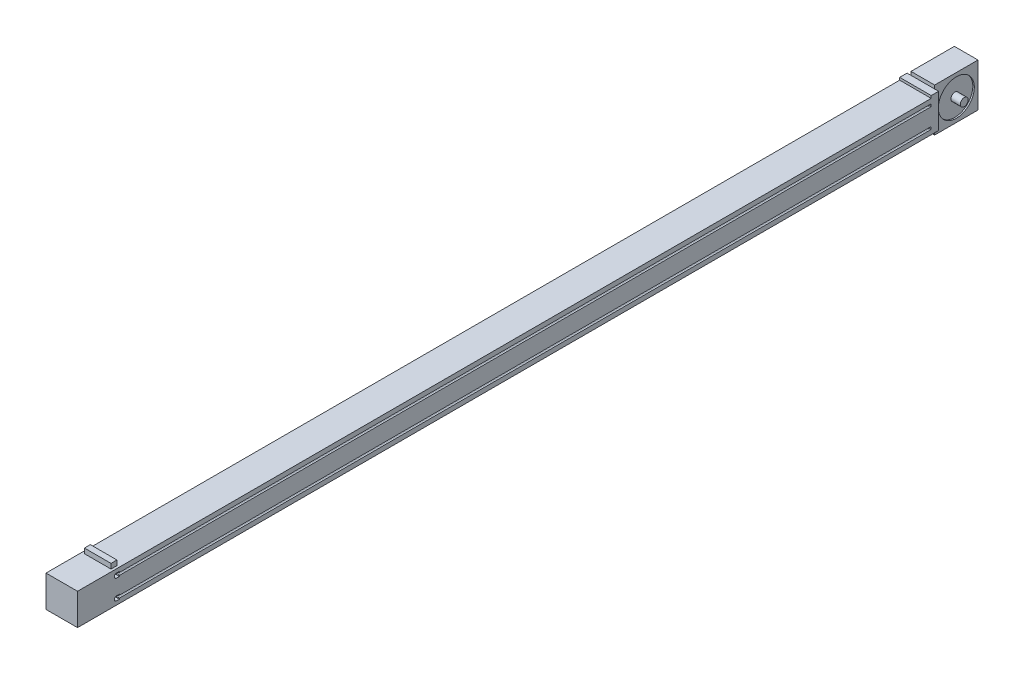
SolidWorks part; units mm, degrees
ref_plane "前视" through (0, 0, 0) normal (0, 0, 1) x (1, 0, 0)
ref_plane "上视" through (0, 0, 0) normal (0, 1, 0) x (1, 0, 0)
ref_plane "右视" through (0, 0, 0) normal (1, 0, 0) x (0, 0, -1)
sketch "草图1" plane through (0, 0, 0) normal (0, 0, 1) x (1, 0, 0)
  line L0 (41.9319, 63.6353) -> (41.9319, -24.9145) construction
  line L1 (9.9319, 6.9259) -> (9.9319, 41.9259)
  line L2 (9.9319, 56.4259) -> (73.9319, 56.4259)
  line L3 (9.9319, 46.9259) -> (12.9319, 46.9259)
  line L4 (1.2009, 24.4259) -> (59.3506, 24.4259) construction
  line L5 (12.9319, 46.9259) -> (12.9319, 48.4259)
  line L6 (12.9319, 48.4259) -> (16.9319, 48.4259)
  line L7 (16.9319, 48.4259) -> (16.9319, 40.4259)
  line L8 (16.9319, 40.4259) -> (12.9319, 40.4259)
  line L9 (12.9319, 40.4259) -> (12.9319, 41.9259)
  line L10 (12.9319, 41.9259) -> (9.9319, 41.9259)
  line L11 (9.9319, 46.9259) -> (9.9319, 56.4259)
  line L12 (9.9319, 1.9259) -> (9.9319, -7.5741)
  line L13 (12.9319, 6.9259) -> (9.9319, 6.9259)
  line L14 (12.9319, 8.4259) -> (12.9319, 6.9259)
  line L15 (16.9319, 8.4259) -> (12.9319, 8.4259)
  line L16 (16.9319, 0.4259) -> (16.9319, 8.4259)
  line L17 (12.9319, 0.4259) -> (16.9319, 0.4259)
  line L18 (12.9319, 1.9259) -> (12.9319, 0.4259)
  line L19 (9.9319, 1.9259) -> (12.9319, 1.9259)
  line L20 (9.9319, -7.5741) -> (73.9319, -7.5741)
  line L21 (73.9319, 1.9259) -> (70.9319, 1.9259)
  line L22 (70.9319, 1.9259) -> (70.9319, 0.4259)
  line L23 (70.9319, 0.4259) -> (66.9319, 0.4259)
  line L24 (66.9319, 0.4259) -> (66.9319, 8.4259)
  line L25 (66.9319, 8.4259) -> (70.9319, 8.4259)
  line L26 (70.9319, 8.4259) -> (70.9319, 6.9259)
  line L27 (70.9319, 6.9259) -> (73.9319, 6.9259)
  line L28 (73.9319, 1.9259) -> (73.9319, -7.5741)
  line L29 (73.9319, 46.9259) -> (73.9319, 56.4259)
  line L30 (70.9319, 41.9259) -> (73.9319, 41.9259)
  line L31 (70.9319, 40.4259) -> (70.9319, 41.9259)
  line L32 (66.9319, 40.4259) -> (70.9319, 40.4259)
  line L33 (66.9319, 48.4259) -> (66.9319, 40.4259)
  line L34 (70.9319, 48.4259) -> (66.9319, 48.4259)
  line L35 (70.9319, 46.9259) -> (70.9319, 48.4259)
  line L36 (73.9319, 46.9259) -> (70.9319, 46.9259)
  line L37 (73.9319, 6.9259) -> (73.9319, 41.9259)
  point P25 (9.9319, 24.4259)
  point P26 (41.9319, -7.5741)
  point P43 (41.9319, 56.4259)
  dimension "D1" = 32
  dimension "D2" = 32
  dimension "D3" = 9.5
  dimension "D4" = 8
  dimension "D5" = 5
  dimension "D6" = 3
  dimension "D7" = 4
extrude "基体-拉伸" add sketch "草图1" against normal blind 1648
sketch "草图2" plane through (0, 0, 0) normal (0, 0, 1) x (1, 0, 0)
  line L1 (73.9319, -7.5741) -> (9.9319, -7.5741)
  line L2 (73.9319, -7.5741) -> (73.9319, 56.4259)
  line L3 (73.9319, 56.4259) -> (9.9319, 56.4259)
  line L4 (9.9319, -7.5741) -> (9.9319, 56.4259)
extrude "凸台-拉伸1" add sketch "草图2" along normal blind 85
sketch "草图4" plane through (0, 56.4259, 0) normal (0, 1, 0) x (-1, 0, 0)
  line L0 (-73.9319, -1648) -> (-73.9319, 85) construction
  line L1 (-68.9319, 0) -> (-14.9319, 0)
  line L2 (-68.9319, 0) -> (-68.9319, 12)
  line L3 (-68.9319, 12) -> (-14.9319, 12)
  line L4 (-14.9319, 0) -> (-14.9319, 12)
  line L5 (-9.9319, -1648) -> (-9.9319, 85) construction
  dimension "D1" = 5
  dimension "D2" = 5
  dimension "D3" = 12
extrude "凸台-拉伸2" add sketch "草图4" along normal blind 10
sketch "草图5" plane through (73.9319, 0, 0) normal (1, 0, 0) x (0, 0, -1)
  line L0 (1648, 46.9259) -> (0, 46.9259) construction
  line L1 (0, 48.9259) -> (-6, 48.9259)
  line L2 (0, 48.9259) -> (0, 39.9259)
  line L3 (0, 39.9259) -> (-6, 39.9259)
  line L4 (-10, 44.9259) -> (-10, 43.9259)
  line L5 (0, 8.9259) -> (-6, 8.9259)
  line L6 (0, 8.9259) -> (0, -0.0741)
  line L7 (0, -0.0741) -> (-6, -0.0741)
  line L8 (-10, 4.9259) -> (-10, 3.9259)
  line L9 (1648, 41.9259) -> (0, 41.9259) construction
  line L10 (0, 41.9259) -> (0, 46.9259) construction
  line L11 (1648, 6.9259) -> (0, 6.9259) construction
  line L12 (1648, 1.9259) -> (0, 1.9259) construction
  line L13 (0, 1.9259) -> (0, 6.9259) construction
  arc A0 (-10, 43.9259) -> (-6, 39.9259) centre (-6, 43.9259) ccw
  arc A1 (-6, 48.9259) -> (-10, 44.9259) centre (-6, 44.9259) ccw
  arc A2 (-10, 4.9259) -> (-6, 8.9259) centre (-6, 4.9259) cw
  arc A3 (-10, 3.9259) -> (-6, -0.0741) centre (-6, 3.9259) ccw
  point P16 (-10, 39.9259)
  point P27 (-10, 8.9259)
  dimension "D4" = 4
  dimension "D5" = 4
  dimension "D9" = 4
  dimension "D1" = 2
  dimension "D2" = 2
  dimension "D3" = 10
  dimension "D6" = 2
  dimension "D7" = 2
  dimension "D8" = 10
extrude "切除-拉伸1" cut sketch "草图5" against normal blind 10
ref_plane "基准面4" through (41.9319, 0, 0) normal (-1, 0, 0) x (0, 0, 1)
mirror "镜向1" about plane through (41.9319, 0, 0) normal (-1, 0, 0) of "切除-拉伸1"
sketch "草图6" plane through (0, 0, -1648) normal (0, 0, -1) x (-1, 0, 0)
  line L0 (-73.9319, 56.4259) -> (-9.9319, 56.4259) construction
  line L1 (-73.9319, -7.5741) -> (-9.9319, -7.5741)
  line L2 (-73.9319, -7.5741) -> (-73.9319, 61.4259)
  line L3 (-73.9319, 61.4259) -> (-9.9319, 61.4259)
  line L4 (-9.9319, -7.5741) -> (-9.9319, 61.4259)
  dimension "D1" = 5
extrude "凸台-拉伸3" add sketch "草图6" along normal blind 15
sketch "草图7" plane through (0, 0, -1663) normal (0, 0, -1) x (-1, 0, 0)
  line L0 (-9.9319, 61.4259) -> (-73.9319, 61.4259) construction
  line L1 (-65.9319, -19.5741) -> (-17.9319, -19.5741)
  line L2 (-65.9319, -19.5741) -> (-65.9319, 68.4259)
  line L3 (-65.9319, 68.4259) -> (-17.9319, 68.4259)
  line L4 (-17.9319, -19.5741) -> (-17.9319, 68.4259)
  line L5 (-73.9319, -7.5741) -> (-9.9319, -7.5741) construction
  line L6 (-73.9319, 61.4259) -> (-73.9319, -7.5741) construction
  line L7 (-9.9319, -7.5741) -> (-9.9319, 61.4259) construction
  dimension "D1" = 7
  dimension "D2" = 12
  dimension "D3" = 8
  dimension "D4" = 8
extrude "凸台-拉伸4" add sketch "草图7" along normal blind 88
sketch "草图8" plane through (17.9319, 0, 0) normal (-1, 0, 0) x (0, 0, 1)
  line L0 (-1751, -19.5741) -> (-1663, -19.5741) construction
  line L2 (-1648, 56.4259) -> (-1648, 61.4259) construction
  circle A0 centre (-1707, 24.4259) radius 36.5
  dimension "D1" = 73
  dimension "D2" = 44
  dimension "D3" = 59
extrude "切除-拉伸2" cut sketch "草图8" against normal blind 3
sketch "草图9" plane through (20.9319, 0, 0) normal (-1, 0, 0) x (0, 0, 1)
  circle A0 centre (-1707, 24.4259) radius 8
  circle A1 centre (-1707, 24.4259) radius 36.5 construction
  dimension "D1" = 16
extrude "凸台-拉伸5" add sketch "草图9" along normal blind 19
mirror "镜向2" about plane through (41.9319, 0, 0) normal (-1, 0, 0) of "凸台-拉伸5", "切除-拉伸2"
